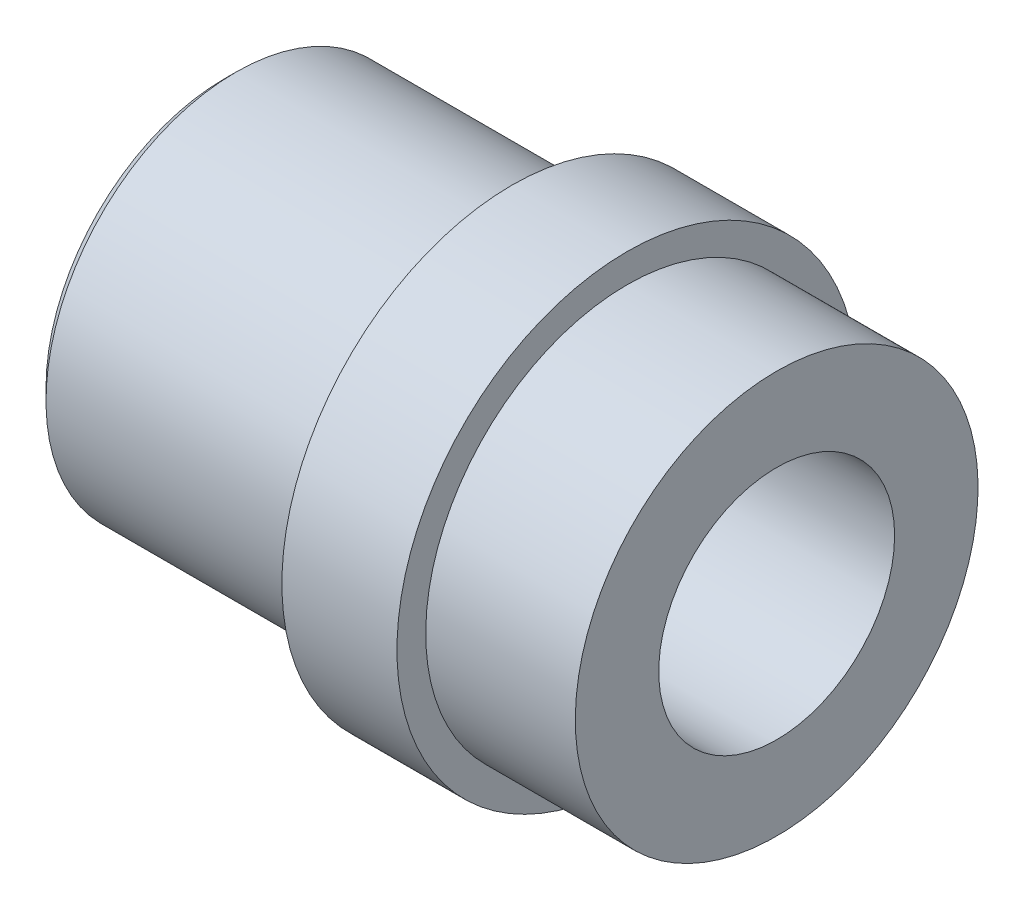
SolidWorks part; units mm, degrees
material "45"
ref_plane "Front Plane" through (0, 0, 0) normal (0, 0, 1) x (1, 0, 0)
ref_plane "Top Plane" through (0, 0, 0) normal (0, 1, 0) x (1, 0, 0)
ref_plane "Right Plane" through (0, 0, 0) normal (1, 0, 0) x (0, 0, -1)
sketch "Sketch1" plane through (0, 0, 0) normal (0, 0, 1) x (1, 0, 0)
  line L0 (0, 0) -> (-25.4468, 0) construction
  line L1 (-48, 0) -> (-48, 15.5)
  line L2 (-47, 16.5) -> (-23, 16.5)
  line L3 (-23, 16.5) -> (-23, 20)
  line L4 (-23, 20) -> (-13, 20)
  line L5 (-13, 20) -> (-13, 17.5)
  line L6 (-13, 17.5) -> (0, 17.5)
  line L7 (0, 17.5) -> (0, 0)
  line L8 (-48, 15.5) -> (-47, 16.5)
  line L9 (-48, 0) -> (0, 0)
  point P4 (-48, 16.5)
  dimension "D1" = 20
  dimension "D2" = 17.5
  dimension "D3" = 16.5
  dimension "D4" = 0
  dimension "D5" = 13
  dimension "D6" = 48
  dimension "D7" = 25
  dimension "D8" = 0
revolve "Revolve1" add sketch "Sketch1" angle 360 about L0
cosmetic thread "Cosmetic Thread1" parameters "D1"=23.9999, "D2"=30.835
sketch "Sketch2" plane through (0, 0, 0) normal (1, 0, 0) x (0, 0, -1)
  circle A0 centre (0, 0) radius 10
  dimension "D1" = 20
extrude "Cut-Extrude1" cut sketch "Sketch2" against normal through all
hole_wizard "M22x1.5 Tapped Hole2" positions "Sketch5" profile "Sketch6" tap size "M22x1.5" standard "GB"
sketch "Sketch5" plane through (0, 0, 0) normal (1, 0, 0) x (0, 0, -1)
  point P0 (0, 0)
sketch "Sketch6" plane through (0, 0, 0) normal (0, 1, 0) x (0, 0, -1)
  line L0 (0, 0) -> (0, 28.1588)
  line L1 (0, 28.1588) -> (10.25, 22)
  line L2 (10.25, 22) -> (10.25, 0)
  line L5 (10.25, 0) -> (0, 0)
  line L10 (0, 28.1588) -> (-10.25, 22) construction
  line L11 (0, -6.35) -> (0, 107.95) construction
  dimension "螺纹孔钻头直径" = 20.5
  dimension "螺纹孔钻头深度" = 22
  dimension "导头角度" = 118
cosmetic thread "Cosmetic thread4"
